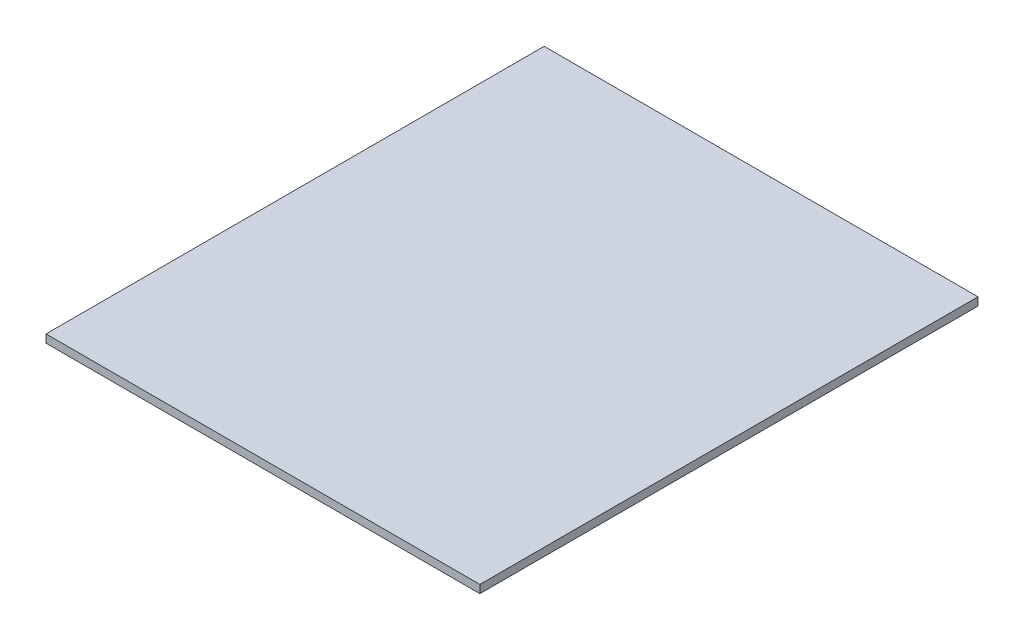
SolidWorks part; units mm, degrees
ref_plane "Front Plane" through (0, 0, 0) normal (0, 0, 1) x (1, 0, 0)
ref_plane "Top Plane" through (0, 0, 0) normal (0, 1, 0) x (1, 0, 0)
ref_plane "Right Plane" through (0, 0, 0) normal (1, 0, 0) x (0, 0, -1)
sketch "Sketch1" plane through (0, 0, 0) normal (0, 1, 0) x (1, 0, 0)
  line L1 (-135, 155) -> (135, 155)
  line L2 (-135, 155) -> (-135, -155)
  line L3 (-135, -155) -> (135, -155)
  line L4 (135, 155) -> (135, -155)
  line L5 (-135, 155) -> (135, -155) construction
  line L6 (-135, -155) -> (135, 155) construction
  point P0 (0, 0)
  dimension "D1" = 270
  dimension "D2" = 310
extrude "Boss-Extrude1" add sketch "Sketch1" along normal blind 5
